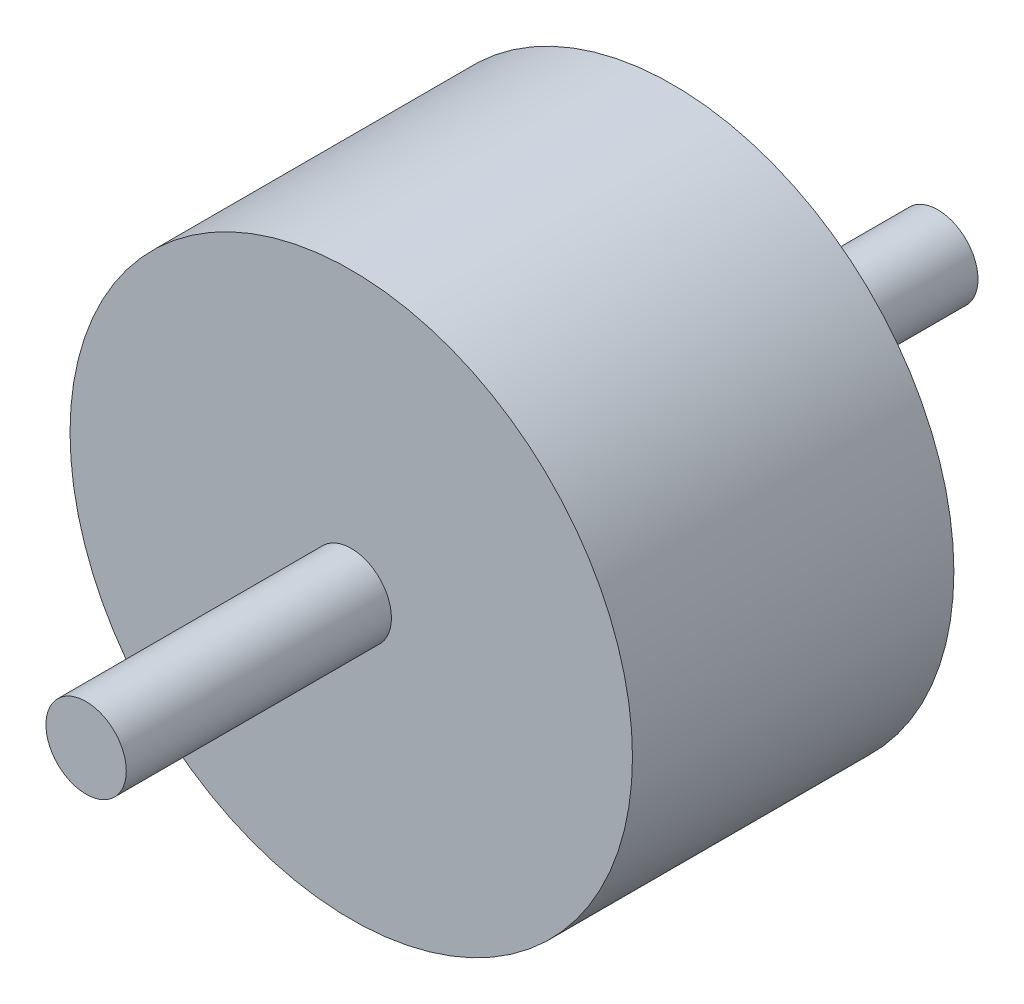
SolidWorks part; units mm, degrees
ref_plane "前视基准面" through (0, 0, 0) normal (0, 0, 1) x (1, 0, 0)
ref_plane "上视基准面" through (0, 0, 0) normal (0, 1, 0) x (1, 0, 0)
ref_plane "右视基准面" through (0, 0, 0) normal (1, 0, 0) x (0, 0, -1)
sketch "草图1" plane through (0, 0, 0) normal (0, 0, 1) x (1, 0, 0)
  circle A0 centre (0, 0) radius 35
  dimension "D1" = 70
extrude "凸台-拉伸1" add sketch "草图1" along normal blind 40
sketch "草图2" plane through (0, 0, 40) normal (0, 0, 1) x (1, 0, 0)
  circle A0 centre (0, 0) radius 5
  dimension "D1" = 10
extrude "凸台-拉伸2" add sketch "草图2" along normal blind 33
sketch "草图3" plane through (0, 0, 0) normal (0, 0, -1) x (-1, 0, 0)
  circle A0 centre (0, 0) radius 5
  dimension "D1" = 10
extrude "凸台-拉伸3" add sketch "草图3" along normal blind 33
